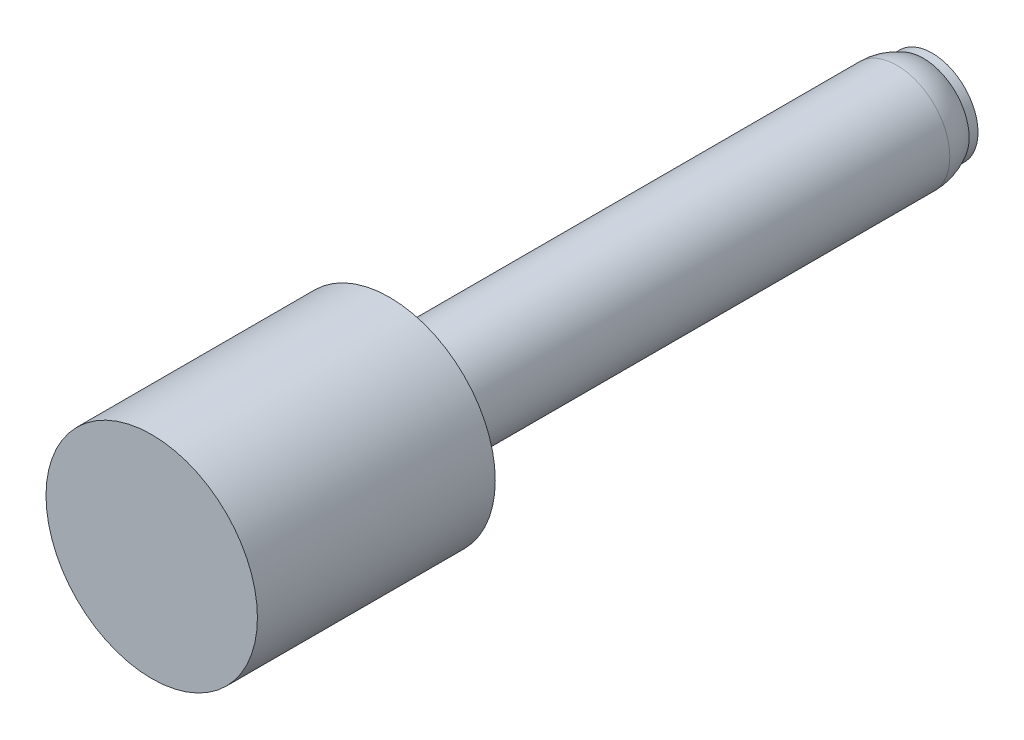
from build123d import *

# Parameters (mm, degrees)
SKETCH1_R           = 60
BOSS_EXTRUDE1_DEPTH = 135
SKETCH2_R           = 30
BOSS_EXTRUDE2_DEPTH = 318
FILLET2_R           = 30
SKETCH3_R           = 26
BOSS_EXTRUDE3_DEPTH = 20


with BuildPart() as part:
    # Sketch1 → Boss-Extrude1 (new body)
    with BuildSketch(Plane.XY):
        with Locations((599.884196758, 0)):
            Circle(SKETCH1_R)
    extrude(amount=-BOSS_EXTRUDE1_DEPTH)

    # Sketch2 → Boss-Extrude2 (add)
    with BuildSketch(Plane(origin=(0, 0, -135), x_dir=(-1, 0, 0), z_dir=(0, 0, -1))):
        with Locations((-599.884196758, 0)):
            Circle(SKETCH2_R)
    extrude(amount=BOSS_EXTRUDE2_DEPTH)

    # Fillet2
    fillet2_edges = [part.edges().sort_by_distance(p)[0] for p in [
        (629.884196758, 0, -453),
    ]]
    fillet(fillet2_edges, radius=FILLET2_R)

    # Sketch3 → Boss-Extrude3 (add)
    with BuildSketch(Plane.XY.offset(-423)):
        with Locations((599.884196758, 0)):
            Circle(SKETCH3_R)
    extrude(amount=-BOSS_EXTRUDE3_DEPTH)


solid = part.part
